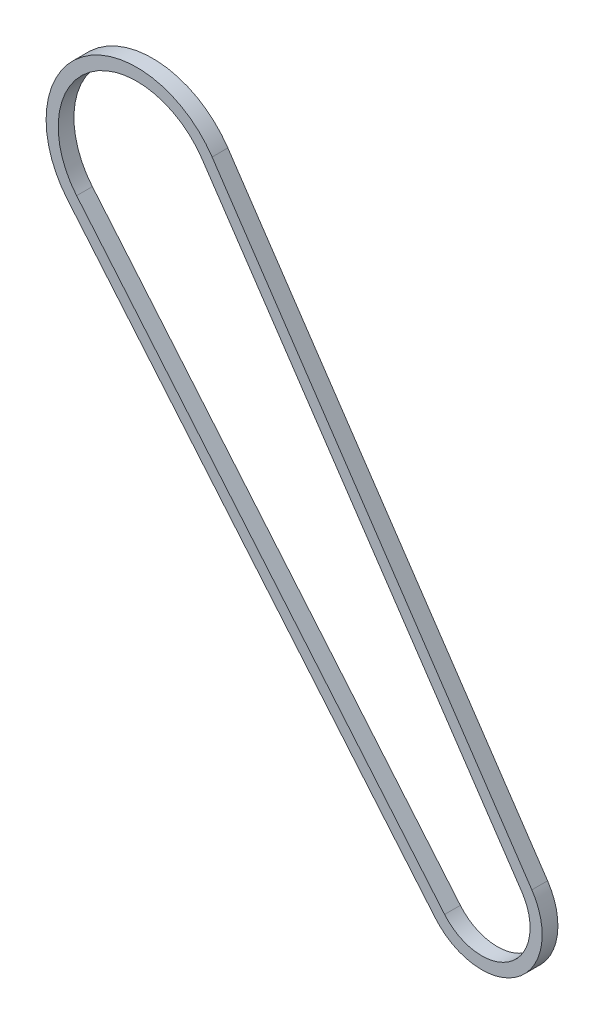
from build123d import *

# Parameters (mm, degrees)
EXTRUDE_THIN1_DEPTH = 6.5


with BuildPart() as part:
    # Sketch2 → Extrude-Thin1 (new, symmetric)
    with BuildSketch(Plane.XY):
        with BuildLine():
            Line((246.701365565, -410.604367651), (-57.447951652, -48.215483519))
            ThreePointArc((-57.447951652, -48.215483519), (-45.116879333, 59.912162365), (62.209431887, 41.892560011))
            Line((62.209431887, 41.892560011), (326.472954592, -350.532338631))
            ThreePointArc((326.472954592, -350.532338631), (315.077919555, -418.402153548), (246.701365565, -410.604367651))
        make_face()
        with BuildLine():
            Line((254.361092452, -404.175636515), (-49.788224765, -41.786752383))
            ThreePointArc((-49.788224765, -41.786752383), (-39.101295422, 51.92387405), (53.914840969, 36.306885343))
            Line((53.914840969, 36.306885343), (318.178363673, -356.118013299))
            ThreePointArc((318.178363673, -356.118013299), (309.062335644, -410.413865233), (254.361092452, -404.175636515))
        make_face(mode=Mode.SUBTRACT)
    extrude(amount=EXTRUDE_THIN1_DEPTH, both=True)


solid = part.part
